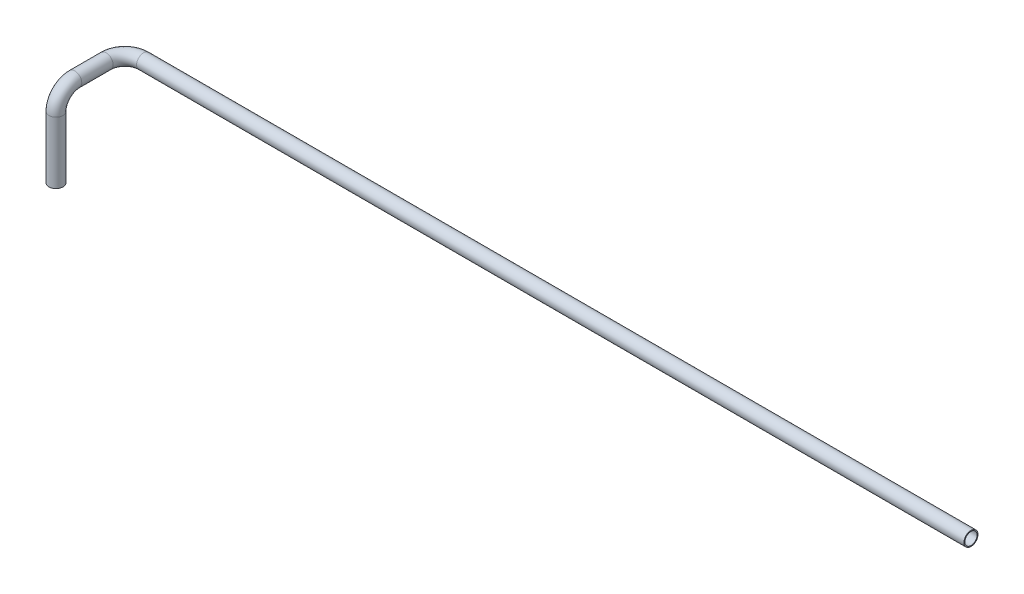
from build123d import *

# Parameters (mm, degrees)
SWEEP_THIN1_PROFILE_R   = 15
SWEEP_THIN1_PROFILE_R_2 = 13


with BuildPart() as part:
    # Sweep-Thin1: sweep along a curve in space
    with BuildLine() as sweep_thin1_path:
        Line((-2200, 3201.170909047, 100), (-2200, 3332.935752391, 100))
        ThreePointArc((-2200, 3332.935752391, 100), (-2200, 3361.220023638, 88.284271247), (-2200, 3372.935752391, 60))
        Line((-2200, 3372.935752391, 60), (-2200, 3372.935752391, -6.776695297))
        ThreePointArc((-2200, 3372.935752391, -6.776695297), (-2188.284271248, 3372.935752391, -35.060966545), (-2160, 3372.935752391, -46.776695297))
        Line((-2160, 3372.935752391, -46.776695297), (-397.65799846, 3372.935752391, -46.776695297))
    # Sweep-Thin1 profile (on start of the path) → Sweep-Thin1 (sweep)
    with BuildSketch(Plane(origin=(-2200, 3201.170909047, 100), x_dir=(0, 0, 1), z_dir=(0, 1, 0))):
        Circle(SWEEP_THIN1_PROFILE_R)
        Circle(SWEEP_THIN1_PROFILE_R_2, mode=Mode.SUBTRACT)
    sweep(path=sweep_thin1_path.line)


solid = part.part
